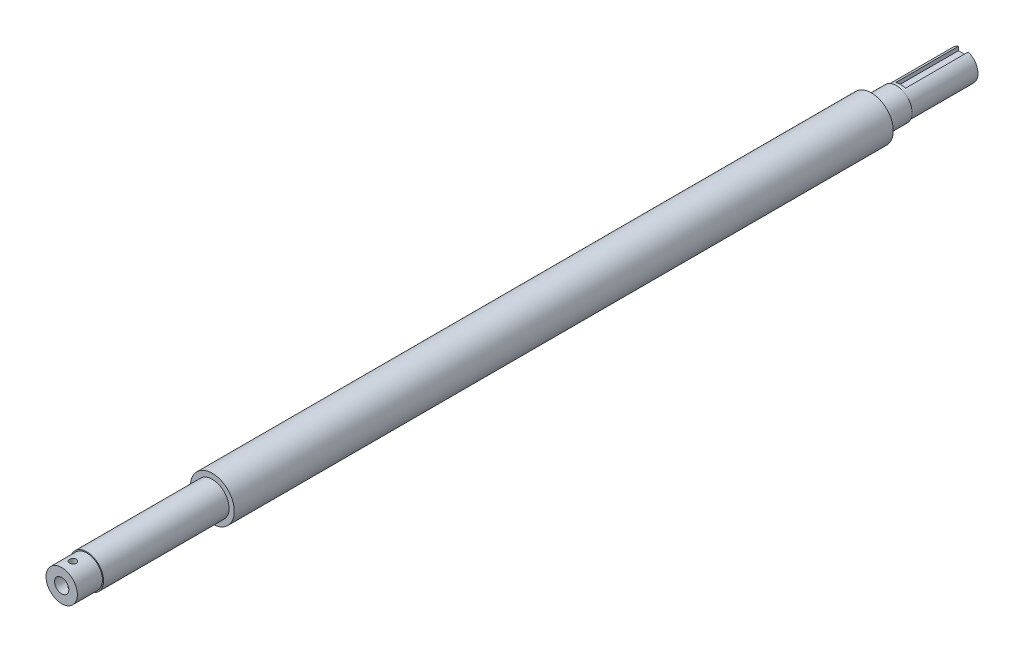
SolidWorks part; units mm, degrees
ref_plane "前视基准面" through (0, 0, 0) normal (0, 0, 1) x (1, 0, 0)
ref_plane "上视基准面" through (0, 0, 0) normal (0, 1, 0) x (1, 0, 0)
ref_plane "右视基准面" through (0, 0, 0) normal (1, 0, 0) x (0, 0, -1)
sketch "草图1" plane through (0, 0, 0) normal (0, 0, 1) x (1, 0, 0)
  circle A0 centre (0, 0) radius 7.5
  dimension "D1" = 15
extrude "凸台-拉伸1" add sketch "草图1" along normal blind 12
sketch "草图2" plane through (0, 0, 0) normal (0, 0, -1) x (-1, 0, 0)
  circle A0 centre (0, 0) radius 8
extrude "凸台-拉伸2" add sketch "草图2" along normal blind 60
sketch "草图3" plane through (0, 0, -60) normal (0, 0, -1) x (-1, 0, 0)
  circle A0 centre (0, 0) radius 10.5
  dimension "D1" = 21
extrude "凸台-拉伸3" add sketch "草图3" along normal blind 315
cosmetic thread "装饰螺纹线1" parameters "D2"=20
sketch "草图4" plane through (0, 0, -375) normal (0, 0, -1) x (-1, 0, 0)
  circle A0 centre (0, 0) radius 7.5
extrude "凸台-拉伸4" add sketch "草图4" along normal blind 12
sketch "草图5" plane through (0, 0, -387) normal (0, 0, -1) x (-1, 0, 0)
  circle A0 centre (0, 0) radius 7
  dimension "D1" = 14
extrude "凸台-拉伸5" add sketch "草图5" along normal blind 32
sketch "草图6" plane through (0, 0, -419) normal (0, 0, -1) x (-1, 0, 0)
  line L1 (2.3537, 9.2415) -> (-2.3537, 9.2415)
  line L2 (2.3537, 9.2415) -> (2.3537, 4.7585)
  line L3 (2.3537, 4.7585) -> (-2.3537, 4.7585)
  line L4 (-2.3537, 9.2415) -> (-2.3537, 4.7585)
  line L5 (2.3537, 9.2415) -> (-2.3537, 4.7585) construction
  line L6 (2.3537, 4.7585) -> (-2.3537, 9.2415) construction
  circle A0 centre (0, 0) radius 7 construction
  point P0 (0, 7)
extrude "切除-拉伸1" cut sketch "草图6" against normal blind 30
hole_wizard "M8 螺纹孔1" positions "草图8" profile "草图7" tap size "M8" standard "Iso"
sketch "草图8" plane through (0, 0, 12) normal (0, 0, 1) x (1, 0, 0)
  point P0 (0, 0)
sketch "草图7" plane through (0, 0, 12) normal (1, 0, 0) x (0, -1, 0)
  line L0 (0, 0) -> (0, 21.7929)
  line L1 (0, 21.7929) -> (3.4, 19.75)
  line L2 (3.4, 19.75) -> (3.4, 0)
  line L5 (3.4, 0) -> (0, 0)
  line L10 (0, 21.7929) -> (-3.4, 19.75) construction
  line L11 (0, -6.35) -> (0, 107.95) construction
  dimension "螺纹孔钻头直径" = 6.8
  dimension "螺纹孔钻头深度" = 19.75
  dimension "导头角度" = 118
cosmetic thread "孔螺蚊线1" parameters "D1"=16, "D2"=8
hole_wizard "M4 螺纹孔1" positions "3D草图1" profile "草图9" tap size "M4" standard "Iso" end condition through all
sketch3d "3D草图1"
  point P0 (-0.011, 7.5, 6.6634)
sketch "草图9" plane through (-0.011, 7.5, 6.6634) normal (0, 0, 1) x (-1, -0.0015, 0)
  line L0 (0, 0) -> (0, 18.0154)
  line L1 (0, 18.0154) -> (1.65, 18.0154)
  line L2 (1.65, 18.0154) -> (1.65, 0)
  line L5 (1.65, 0) -> (0, 0)
  line L11 (0, -6.35) -> (0, 107.95) construction
  dimension "通孔螺纹孔钻头直径" = 3.3
  dimension "通孔螺纹孔钻头深度" = 18.0154
cosmetic thread "孔螺蚊线2" parameters "D2"=4
